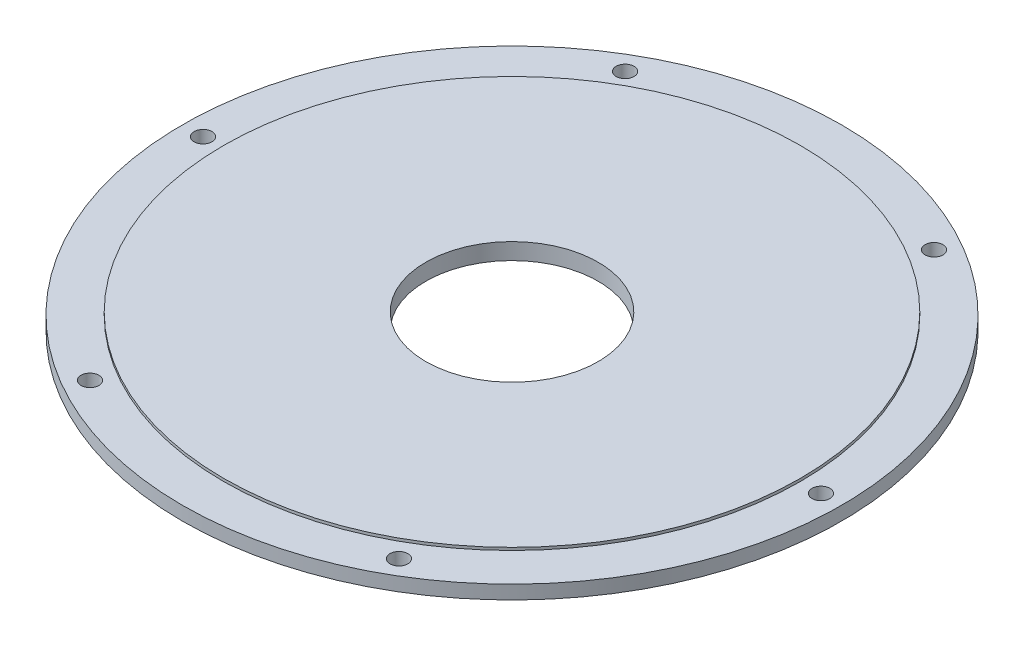
SolidWorks part; units mm, degrees
material "Q235B"
ref_plane "Front Plane" through (0, 0, 0) normal (0, 0, 1) x (1, 0, 0)
ref_plane "Top Plane" through (0, 0, 0) normal (0, 1, 0) x (1, 0, 0)
ref_plane "Right Plane" through (0, 0, 0) normal (1, 0, 0) x (0, 0, -1)
sketch "Sketch1" plane through (0, 0, 0) normal (0, 1, 0) x (1, 0, 0)
  circle A0 centre (0, 0) radius 240
  circle A1 centre (0, 0) radius 62.75
  dimension "D1" = 480
  dimension "D2" = 125.5
extrude "Boss-Extrude1" add sketch "Sketch1" along normal mid plane 12
hole_wizard "Ø13.0 (13) Diameter Hole1" positions "Sketch2" profile "Sketch3" hole size "Ø13.0" standard "GB" end condition up to next
sketch "Sketch2" plane through (0, 6, 0) normal (0, 1, 0) x (1, 0, 0)
  line L0 (0, 0) -> (0, 225) construction
  circle A0 centre (0, 0) radius 225 construction
  point P0 (112.5, -194.8557)
  point P73 (-112.5, -194.8557)
  point P74 (-225, 0)
  point P75 (-112.5, 194.8557)
  point P76 (112.5, 194.8557)
  point P77 (225, 0)
  dimension "D1" = 450
  dimension "D2" = 6
sketch "Sketch3" plane through (112.5, 6, 194.8557) normal (1, 0, 0) x (0, 0, 1)
  line L0 (0, 0) -> (0, 12)
  line L1 (0, 12) -> (6.5, 12)
  line L2 (6.5, 12) -> (6.5, 0)
  line L5 (6.5, 0) -> (0, 0)
  line L11 (0, -6.35) -> (0, 107.95) construction
  dimension "通孔孔直径" = 13
  dimension "通孔孔深度" = 12
sketch "Sketch4" plane through (0, 6, 0) normal (0, 1, 0) x (1, 0, 0)
  circle A0 centre (0, 0) radius 210
  dimension "D1" = 420
extrude "Cut-Extrude1" cut sketch "Sketch4" against normal blind 2 flip side to cut
